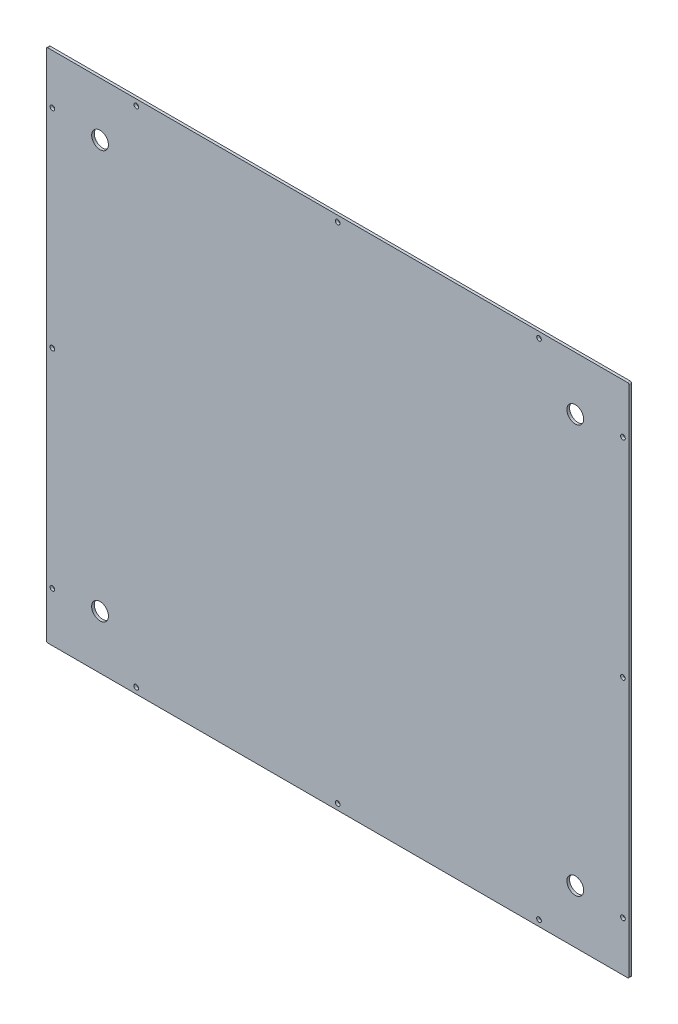
SolidWorks part; units mm, degrees
ref_plane "前视基准面" through (0, 0, 0) normal (0, 0, 1) x (1, 0, 0)
ref_plane "上视基准面" through (0, 0, 0) normal (0, 1, 0) x (1, 0, 0)
ref_plane "右视基准面" through (0, 0, 0) normal (1, 0, 0) x (0, 0, -1)
sketch "草图1" plane through (0, 0, 0) normal (0, 0, 1) x (1, 0, 0)
  line L1 (434, -384) -> (-434, -384)
  line L2 (434, -384) -> (434, 384)
  line L3 (434, 384) -> (-434, 384)
  line L4 (-434, -384) -> (-434, 384)
  line L5 (434, -384) -> (-434, 384) construction
  line L6 (434, 384) -> (-434, -384) construction
  point P0 (0, 0)
  dimension "D1" = 868
  dimension "D2" = 768
extrude "凸台-拉伸1" add sketch "草图1" along normal blind 4
fillet "圆角1" radius 2 4 edges at (434, 384, 2) (434, -384, 2) (-434, -384, 2) (-434, 384, 2)
hole_wizard "M6 间隙孔1" positions "草图3" profile "草图4" hole size "M6" standard "GB" end condition up to next
sketch "草图3" plane through (0, 0, 4) normal (0, 0, 1) x (1, 0, 0)
  line L0 (-425, 310) -> (-425, -310) construction
  line L3 (-434, 0) -> (-425, 0) construction
  line L4 (-434, 382) -> (-434, -382) construction
  point P0 (-425, 310)
  point P2 (-425, -310)
  point P10 (-425, 0)
  dimension "D1" = 620
  dimension "D2" = 9
sketch "草图4" plane through (-425, 310, 4) normal (1, 0, 0) x (0, -1, 0)
  line L0 (0, 0) -> (0, 4)
  line L1 (0, 4) -> (3.5, 4)
  line L2 (3.5, 4) -> (3.5, 0)
  line L5 (3.5, 0) -> (0, 0)
  line L11 (0, -6.35) -> (0, 107.95) construction
  dimension "通孔孔直径" = 7
  dimension "通孔孔深度" = 4
mirror "镜向2" about plane through (0, 0, 0) normal (1, 0, 0) of "M6 间隙孔1"
hole_wizard "M6 间隙孔2" positions "草图5" profile "草图6" hole size "M6" standard "GB" end condition up to next
sketch "草图5" plane through (0, 0, 4) normal (0, 0, 1) x (1, 0, 0)
  line L0 (-300, 375) -> (300, 375) construction
  line L3 (0, 375) -> (0, 384) construction
  line L4 (432, 384) -> (-432, 384) construction
  point P0 (-300, 375)
  point P2 (300, 375)
  point P11 (0, 375)
  dimension "D1" = 9
  dimension "D2" = 600
sketch "草图6" plane through (-300, 375, 4) normal (1, 0, 0) x (0, -1, 0)
  line L0 (0, 0) -> (0, 4)
  line L1 (0, 4) -> (3.5, 4)
  line L2 (3.5, 4) -> (3.5, 0)
  line L5 (3.5, 0) -> (0, 0)
  line L11 (0, -6.35) -> (0, 107.95) construction
  dimension "通孔孔直径" = 7
  dimension "通孔孔深度" = 4
mirror "镜向3" about plane through (0, 0, 0) normal (0, 1, 0) of "M6 间隙孔2"
sketch "草图7" plane through (0, 0, 4) normal (0, 0, 1) x (1, 0, 0)
  line L0 (-432, -384) -> (432, -384) construction
  line L1 (-434, 382) -> (-434, -382) construction
  circle A0 centre (-354, -304) radius 12.5
  dimension "D1" = 25
  dimension "D2" = 80
  dimension "D3" = 80
extrude "切除-拉伸1" cut sketch "草图7" against normal up to next
mirror "镜向4" about plane through (0, 0, 0) normal (1, 0, 0) of "切除-拉伸1"
mirror "镜向5" about plane through (0, 0, 0) normal (0, 1, 0) of "镜向4", "切除-拉伸1"
